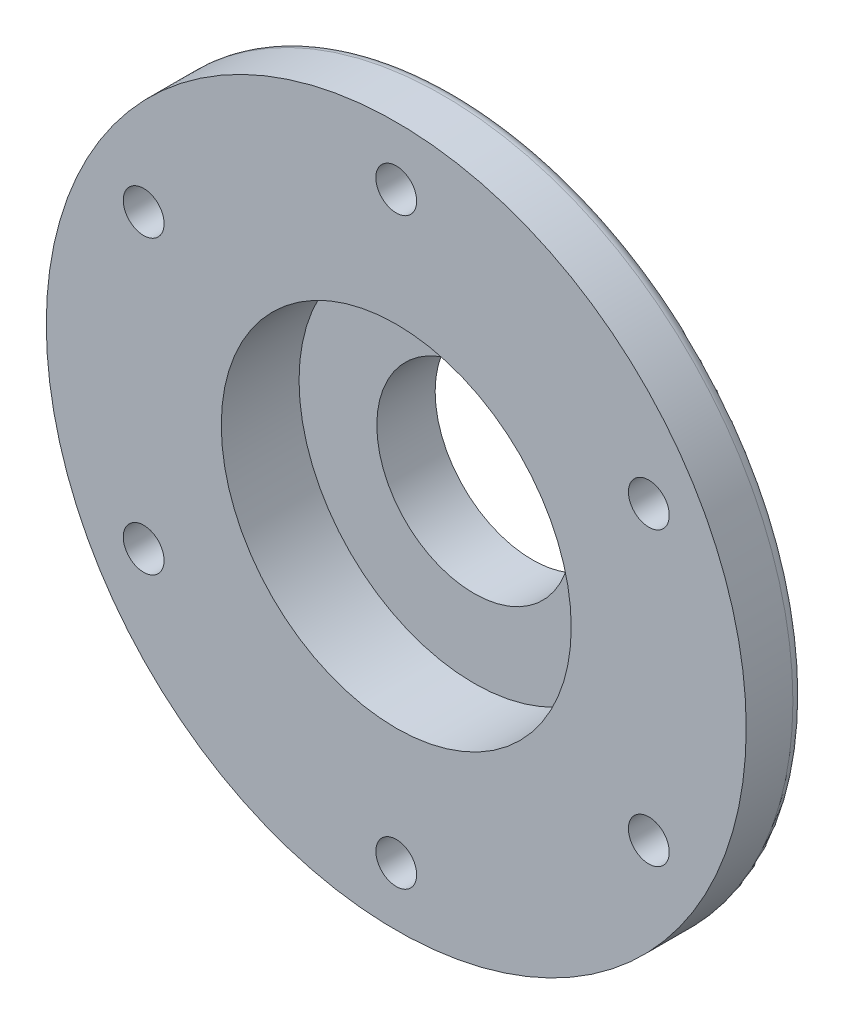
from build123d import *
from build123d.topology import SkipClean

# Parameters (mm, degrees)
SKETCH_1_R          = 90
SKETCH_1_R_2        = 25
SKETCH_1_R_3        = 5.25
EXTRUDE_1_DEPTH     = 15
EXTRUDE_START       = 20
SKETCH_2_R          = 55
SKETCH_2_R_2        = 25
EXTRUDE_2_DEPTH     = 20
SKETCH_3_R          = 45
CUT_EXTRUDE_1_DEPTH = 20
FILLET_1_R          = 3


with BuildPart() as part:
    # 草图1 → 凸台-拉伸1 (new body)
    with BuildSketch(Plane.XY):
        Circle(SKETCH_1_R)
        Circle(SKETCH_1_R_2, mode=Mode.SUBTRACT)
        with Locations((0, 75)):
            Circle(SKETCH_1_R_3, mode=Mode.SUBTRACT)
        with Locations((64.951905284, 37.5)):
            Circle(SKETCH_1_R_3, mode=Mode.SUBTRACT)
        with Locations((64.951905284, -37.5)):
            Circle(SKETCH_1_R_3, mode=Mode.SUBTRACT)
        with Locations((0, -75)):
            Circle(SKETCH_1_R_3, mode=Mode.SUBTRACT)
        with Locations((-64.951905284, -37.5)):
            Circle(SKETCH_1_R_3, mode=Mode.SUBTRACT)
        with Locations((-64.951905284, 37.5)):
            Circle(SKETCH_1_R_3, mode=Mode.SUBTRACT)
    extrude(amount=EXTRUDE_1_DEPTH)

    # 草图2 → 凸台-拉伸2 (add)
    with SkipClean():  # the faces are left unmerged after this step: merging them gives an invalid solid
        with BuildSketch(Plane(origin=(0, 0, 0), x_dir=(-1, 0, 0), z_dir=(0, 0, -1)).offset(EXTRUDE_START)):
            with Locations(Location((0, 0, 0), (0, 0, 180))):
                Circle(SKETCH_2_R)
            Circle(SKETCH_2_R_2, mode=Mode.SUBTRACT)
        extrude(amount=-EXTRUDE_2_DEPTH)

    # 草图3 → 切除-拉伸1 (cut)
    with BuildSketch(Plane.XY.offset(15)):
        Circle(SKETCH_3_R)
    extrude(amount=-CUT_EXTRUDE_1_DEPTH, mode=Mode.SUBTRACT)

    # 圆角1
    fillet_1_edges = [part.edges().sort_by_distance(p)[0] for p in [
        (-90, 0, 0),
        (-55, 0, 0),
        (-55, 0, -20),
    ]]
    fillet(fillet_1_edges, radius=FILLET_1_R)


solid = part.part
